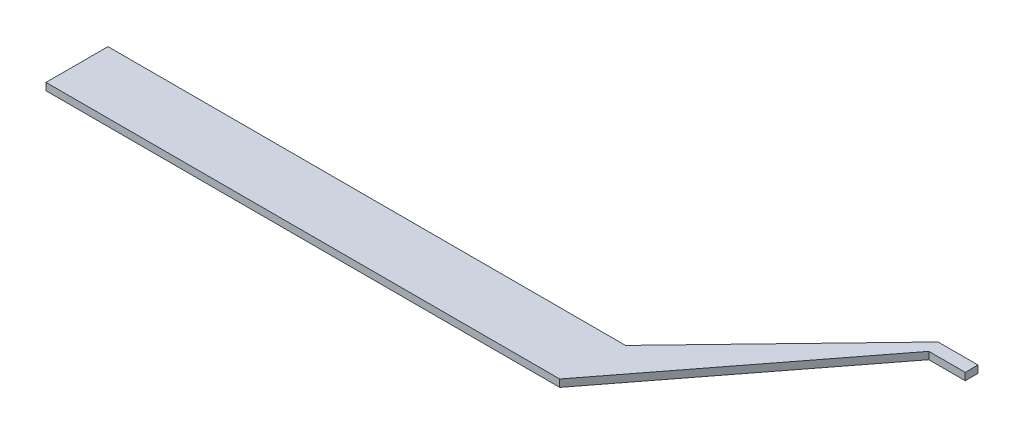
SolidWorks part; units mm, degrees
ref_plane "Front Plane" through (0, 0, 0) normal (0, 0, 1) x (1, 0, 0)
ref_plane "Top Plane" through (0, 0, 0) normal (0, 1, 0) x (1, 0, 0)
ref_plane "Right Plane" through (0, 0, 0) normal (1, 0, 0) x (0, 0, -1)
sketch "Sketch1" plane through (0, 0, 0) normal (0, 1, 0) x (1, 0, 0)
  line L0 (14.2, 1.7) -> (18.4053, 6.07)
  line L1 (0, 0) -> (14.095, 0)
  line L2 (0, 0) -> (0, 1.7)
  line L3 (18.4053, 6.07) -> (19.5, 6.07)
  line L4 (19.5, 5.72) -> (19.5, 6.07)
  line L5 (14.095, 0) -> (18.5, 5.72)
  line L6 (18.5, 5.72) -> (19.5, 5.72)
  line L7 (0, 1.7) -> (14.2, 1.7)
  dimension "D1" = 19.5
  dimension "D2" = 6.07
  dimension "D3" = 1.7
  dimension "D4" = 0.35
  dimension "D5" = 5.3
  dimension "D6" = 52.4
  dimension "D7" = 46.1
  dimension "D8" = 1
extrude "Boss-Extrude1" add sketch "Sketch1" along normal blind 0.2
